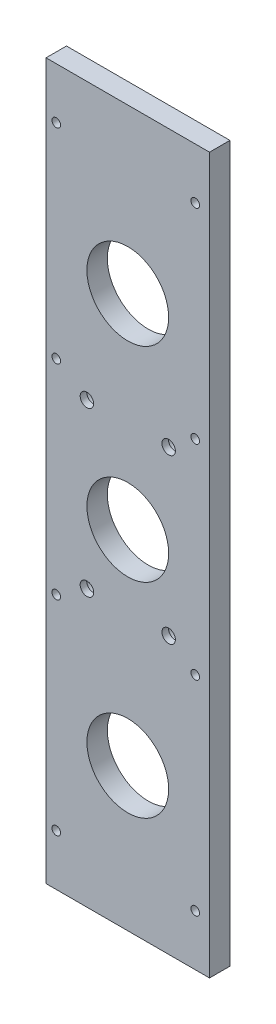
from build123d import *

# Parameters (mm, degrees)
SKETCH_1_W                = 80
SKETCH_1_H                = 350
EXTRUDE_1_DEPTH           = 10
HOLE_WIZARD_M5_1_D        = 4.2
HOLE_WIZARD_1_D           = 6.6
HOLE_WIZARD_1_CBORE_D     = 11
HOLE_WIZARD_1_CBORE_DEPTH = 6.8
CUT_EXTRUDE_1_REACH       = 181.792
SKETCH_6_R                = 20
PATTERN_LINEAR_1_COUNT    = 3
PATTERN_LINEAR_1_PITCH    = 100


with BuildPart() as part:
    # 草图1 → 凸台-拉伸1 (new body)
    with BuildSketch(Plane.XY):
        Rectangle(SKETCH_1_W, SKETCH_1_H)
    extrude(amount=EXTRUDE_1_DEPTH)

    # M5 螺纹孔1 (through all)
    with Locations(Plane(origin=(0, 0, 0), x_dir=(-1, 0, 0), z_dir=(0, 0, -1))):
        with Locations((-33.000000411, 150), (34.999999589, 150), (-33.000000411, 50), (34.999999589, 50), (-33.000000411, -50), (34.999999589, -50), (-33.000000411, -150), (34.999999589, -150)):
            Hole(HOLE_WIZARD_M5_1_D / 2)

    # 打孔尺寸(%根据)内六角圆柱头螺钉的类型1 (through all)
    with Locations(Plane(origin=(0, 0, 0), x_dir=(-1, 0, 0), z_dir=(0, 0, -1))):
        with Locations((-20, 40), (20, 40), (20, -40), (-20, -40)):
            CounterBoreHole(HOLE_WIZARD_1_D / 2, HOLE_WIZARD_1_CBORE_D / 2, HOLE_WIZARD_1_CBORE_DEPTH)

    # 草图6 → 切除-拉伸1 (cut, up to next)
    with BuildSketch(Plane(origin=(0, 0, 0), x_dir=(-1, 0, 0), z_dir=(0, 0, -1)), mode=Mode.PRIVATE) as cut_extrude_1_sk1:
        with Locations((0, -105)):
            Circle(SKETCH_6_R)
    cut_extrude_1_tool1 = extrude(cut_extrude_1_sk1.sketch, amount=-CUT_EXTRUDE_1_REACH, mode=Mode.PRIVATE) & part.part
    cut_extrude_1 = cut_extrude_1_tool1.solids().sort_by_distance((0, -105, 0))[0]
    add(cut_extrude_1, mode=Mode.SUBTRACT)

    # 阵列(线性)1: 切除-拉伸1 ×3
    with Locations(*[(0, i * PATTERN_LINEAR_1_PITCH, 0) for i in range(1, PATTERN_LINEAR_1_COUNT)]):
        add(cut_extrude_1, mode=Mode.SUBTRACT)


solid = part.part
